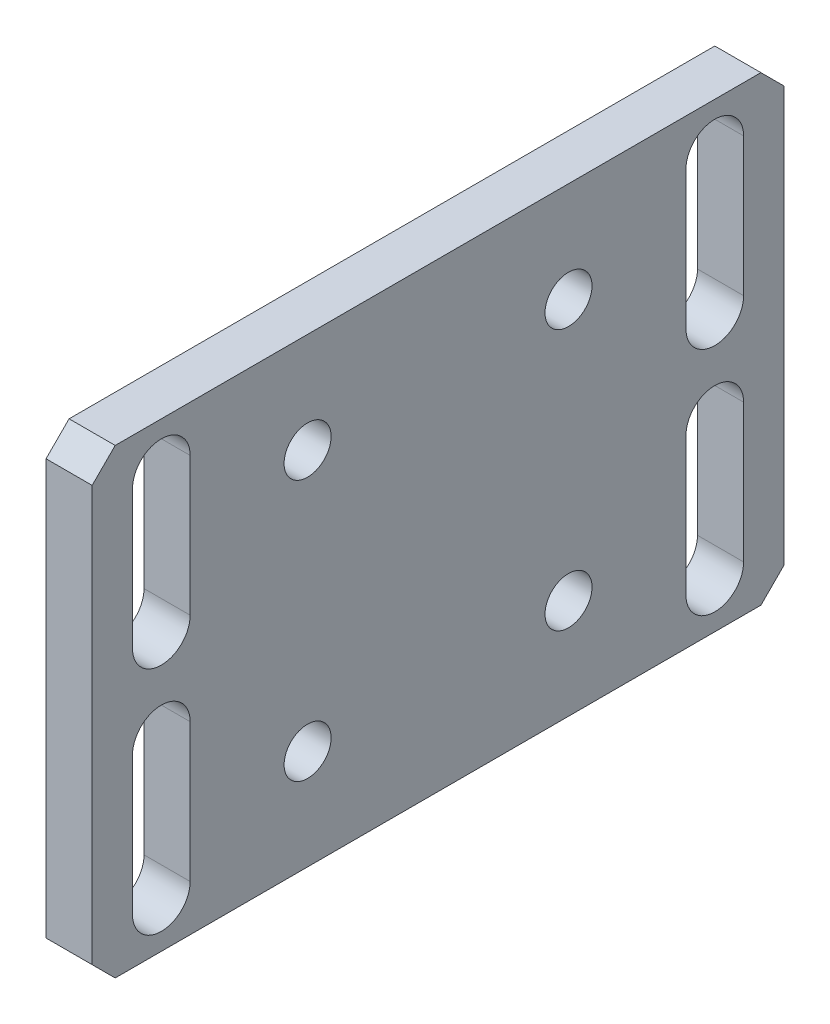
from build123d import *

# Parameters (mm, degrees)
SKETCH_1_W          = 150
SKETCH_1_H          = 100
EXTRUDE_1_DEPTH     = 10
HOLE_WIZARD_M12_1_D = 10.2
CUT_EXTRUDE_1_DEPTH = 91.691785736
CHAMFER_1_SIZE      = 5


with BuildPart() as part:
    # 草图1 → 凸台-拉伸1 (new body)
    with BuildSketch(Plane(origin=(0, 0, 0), x_dir=(0, 0, -1), z_dir=(1, 0, 0))):
        Rectangle(SKETCH_1_W, SKETCH_1_H)
    extrude(amount=EXTRUDE_1_DEPTH)

    # M12 螺纹孔1 (through all)
    with Locations(Plane(origin=(10, 0, 0), x_dir=(0, 0, -1), z_dir=(1, 0, 0))):
        with Locations((-28.284271247, 28.284271247), (28.284271247, 28.284271247), (28.284271247, -28.284271247), (-28.284271247, -28.284271247)):
            Hole(HOLE_WIZARD_M12_1_D / 2)

    # 草图4 → 切除-拉伸1 (cut, through all)
    with BuildSketch(Plane(origin=(10, 0, 0), x_dir=(0, 0, -1), z_dir=(1, 0, 0))):
        with BuildLine():
            Line((-53.75, 40), (-53.75, 10))
            ThreePointArc((-53.75, 10), (-60, 3.75), (-66.25, 10))
            Line((-66.25, 10), (-66.25, 40))
            ThreePointArc((-66.25, 40), (-60, 46.25), (-53.75, 40))
        make_face()
        with BuildLine():
            Line((53.75, 40), (53.75, 10))
            ThreePointArc((53.75, 10), (60, 3.75), (66.25, 10))
            Line((66.25, 10), (66.25, 40))
            ThreePointArc((66.25, 40), (60, 46.25), (53.75, 40))
        make_face()
        with BuildLine():
            Line((-53.75, -40), (-53.75, -10))
            ThreePointArc((-53.75, -10), (-60, -3.75), (-66.25, -10))
            Line((-66.25, -10), (-66.25, -40))
            ThreePointArc((-66.25, -40), (-60, -46.25), (-53.75, -40))
        make_face()
        with BuildLine():
            Line((53.75, -40), (53.75, -10))
            ThreePointArc((53.75, -10), (60, -3.75), (66.25, -10))
            Line((66.25, -10), (66.25, -40))
            ThreePointArc((66.25, -40), (60, -46.25), (53.75, -40))
        make_face()
    extrude(amount=-CUT_EXTRUDE_1_DEPTH, mode=Mode.SUBTRACT)

    # 倒角1
    chamfer_1_edges = [part.edges().sort_by_distance(p)[0] for p in [
        (5, -50, -75),
        (5, -50, 75),
        (5, 50, 75),
        (5, 50, -75),
    ]]
    chamfer(chamfer_1_edges, length=CHAMFER_1_SIZE)


solid = part.part
